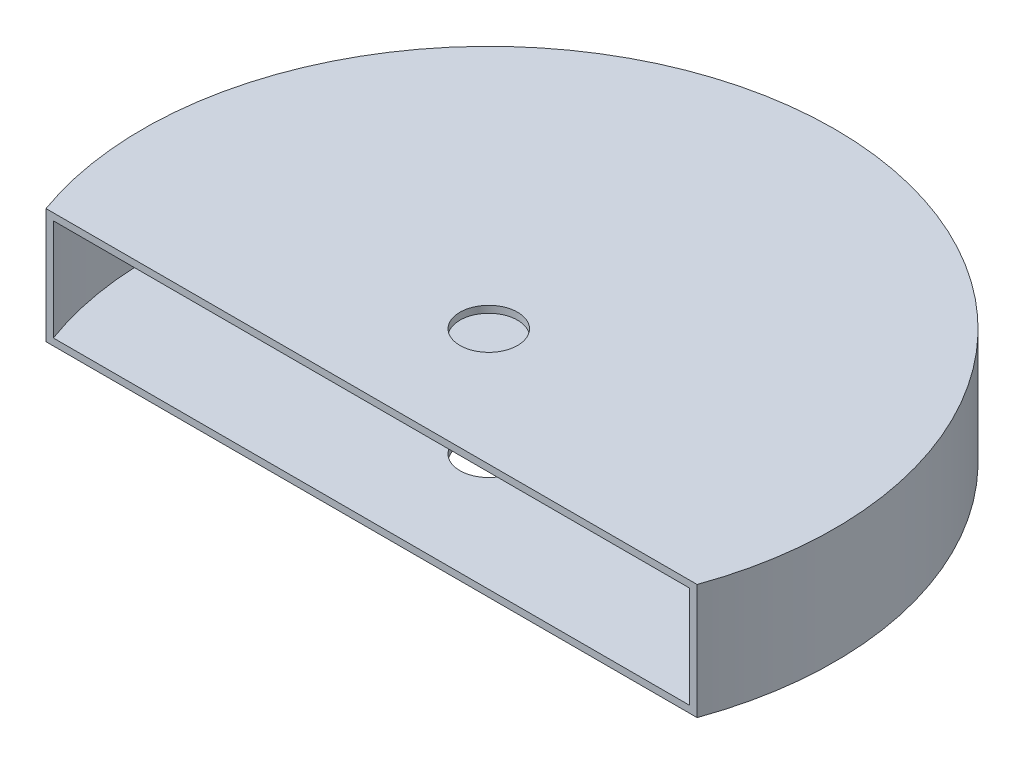
SolidWorks part; units mm, degrees
ref_plane "Front Plane" through (0, 0, 0) normal (0, 0, 1) x (1, 0, 0)
ref_plane "Top Plane" through (0, 0, 0) normal (0, 1, 0) x (1, 0, 0)
ref_plane "Right Plane" through (0, 0, 0) normal (1, 0, 0) x (0, 0, -1)
other "Configuration Table"
sketch "Sketch1" plane through (0, 0, 0) normal (0, 1, 0) x (1, 0, 0)
  line L0 (-141.1309, -50.8142) -> (141.1309, -50.8142)
  arc A1 (141.1309, -50.8142) -> (-141.1309, -50.8142) centre (0, 0) ccw
  dimension "D2" = 300
extrude "Boss-Extrude1" add sketch "Sketch1" along normal blind 50
shell "Shell1" thickness 3
sketch "Sketch2" plane through (0, 50, 0) normal (0, 1, 0) x (1, 0, 0)
  circle A0 centre (0, 0) radius 12.5
  dimension "D1" = 25
extrude "Cut-Extrude1" cut sketch "Sketch2" against normal through all both and the other way through all
